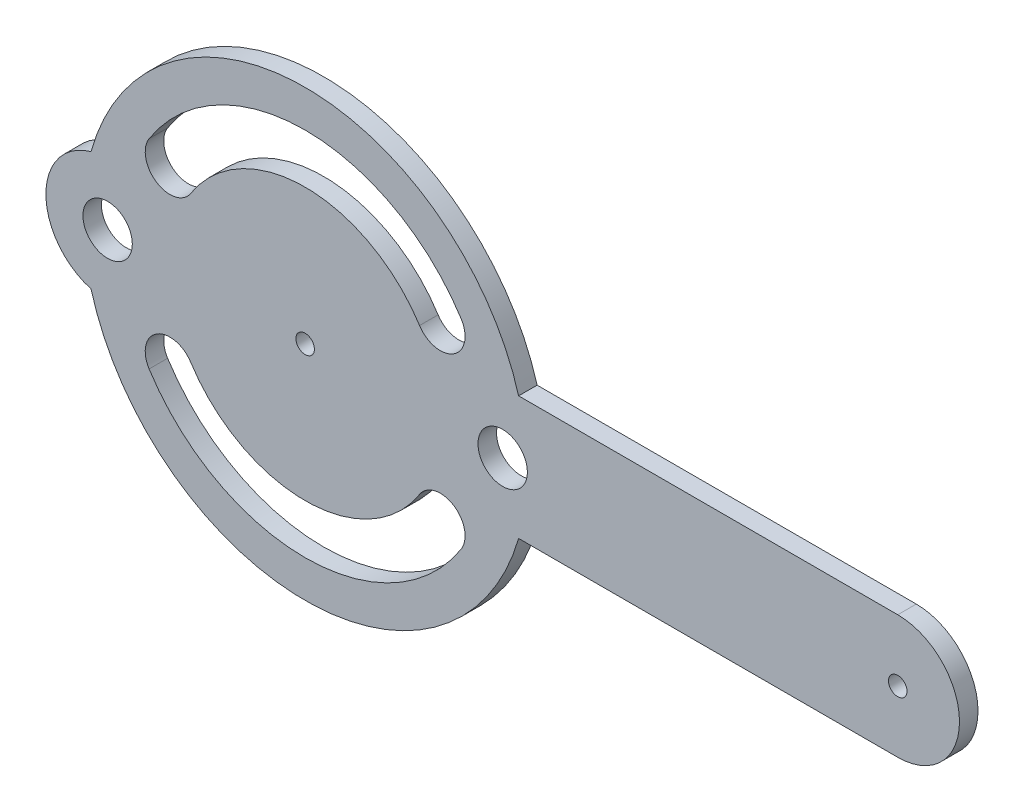
from build123d import *

# Parameters (mm, degrees)
SKETCH_1_R           = 0.75
SKETCH_1_R_2         = 2
BOSS_EXTRUDE_1_DEPTH = 1.5


with BuildPart() as part:
    # Sketch 1 → Boss-Extrude 1 (new body)
    with BuildSketch(Plane.XY):
        with BuildLine():
            Line((48, -5), (17.291616466, -5))
            ThreePointArc((17.291616466, -5), (-0.095597557, -17.99974614), (-17.34375, -4.816049827))
            ThreePointArc((-17.34375, -4.816049827), (-21, 0), (-17.34375, 4.816049827))
            ThreePointArc((-17.34375, 4.816049827), (-0.095597557, 17.99974614), (17.291616466, 5))
            Line((17.291616466, 5), (48, 5))
            ThreePointArc((48, 5), (53, 0), (48, -5))
        make_face()
        Circle(SKETCH_1_R, mode=Mode.SUBTRACT)
        with Locations((16, 0)):
            Circle(SKETCH_1_R_2, mode=Mode.SUBTRACT)
        with Locations((-16, 0)):
            Circle(SKETCH_1_R_2, mode=Mode.SUBTRACT)
        with Locations((48, 0)):
            Circle(SKETCH_1_R, mode=Mode.SUBTRACT)
        with BuildLine():
            ThreePointArc((9.269044534, 5.923243489), (0, 11), (-9.269044534, 5.923243489))
            ThreePointArc((-9.269044534, 5.923243489), (-12.03127872, 5.314916026), (-12.639606182, 8.077150212))
            ThreePointArc((-12.639606182, 8.077150212), (0, 15), (12.639606182, 8.077150212))
            ThreePointArc((12.639606182, 8.077150212), (12.03127872, 5.314916026), (9.269044534, 5.923243489))
        make_face(mode=Mode.SUBTRACT)
        with BuildLine():
            ThreePointArc((-9.269044534, -5.923243489), (-12.03127872, -5.314916026), (-12.639606182, -8.077150212))
            ThreePointArc((-12.639606182, -8.077150212), (0, -15), (12.639606182, -8.077150212))
            ThreePointArc((12.639606182, -8.077150212), (12.03127872, -5.314916026), (9.269044534, -5.923243489))
            ThreePointArc((9.269044534, -5.923243489), (0, -11), (-9.269044534, -5.923243489))
        make_face(mode=Mode.SUBTRACT)
    extrude(amount=BOSS_EXTRUDE_1_DEPTH)


solid = part.part
